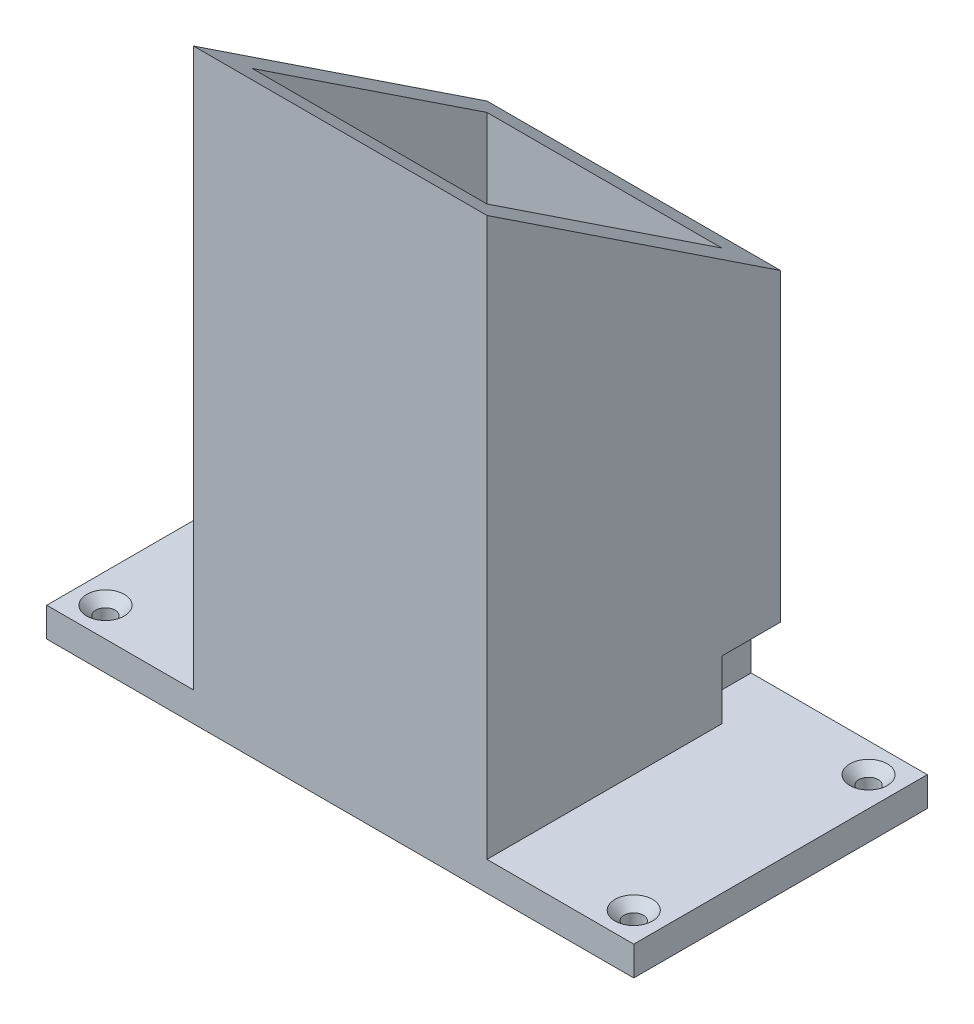
SolidWorks part; units mm, degrees
ref_plane "Front Plane" through (0, 0, 0) normal (0, 0, 1) x (1, 0, 0)
ref_plane "Top Plane" through (0, 0, 0) normal (0, 1, 0) x (1, 0, 0)
ref_plane "Right Plane" through (0, 0, 0) normal (1, 0, 0) x (0, 0, -1)
sketch "Sketch1" plane through (0, 0, 0) normal (0, 0, 1) x (1, 0, 0)
  line L0 (-100, -100) -> (-100, -90)
  line L5 (-50, 100) -> (50, 100)
  line L6 (-50, 100) -> (-50, -100)
  line L7 (-50, -100) -> (50, -100)
  line L8 (50, 100) -> (50, -100)
  line L9 (0, -100) -> (0, 100) construction
  line L10 (-50, 0) -> (50, 0) construction
  line L11 (50, -100) -> (100, -100)
  line L13 (50, -90) -> (100, -90)
  line L14 (100, -100) -> (100, -90)
  line L15 (-50, -100) -> (-100, -100)
  line L16 (-50, -90) -> (-100, -90)
  point P0 (0, 0)
  dimension "D1" = 200
  dimension "D2" = 100
  dimension "D3" = 50
  dimension "D4" = 10
extrude "Boss-Extrude1" add sketch "Sketch1" along normal blind 100 contours L6 L16 L0 L15 | L8 L5 L6 L7 | L11 L14 L13 L8
sketch "Sketch5" plane through (0, 0, 0) normal (1, 0, 0) x (0, 0, -1)
  line L0 (-100, 100) -> (0, 33.7713)
  line L1 (0, 100) -> (0, -90) construction
extrude "Cut-Extrude1" cut sketch "Sketch5" against normal through all and the other way through all
sketch "Sketch7" plane through (0, 0, 0) normal (0, 1, 0) x (1, 0, 0)
  line L0 (-50, -50) -> (50, -50) construction
  line L1 (-50, 0) -> (-50, -100) construction
  line L2 (50, -100) -> (50, 0) construction
  line L3 (0, 0) -> (0, -100) construction
  line L4 (-50, -100) -> (50, -100) construction
  line L5 (50, 0) -> (50, -100) construction
  line L6 (-40, -10) -> (40, -10)
  line L7 (-40, -10) -> (-40, -90)
  line L8 (-40, -90) -> (40, -90)
  line L9 (40, -10) -> (40, -90)
  line L10 (0, -90) -> (0, -10) construction
  line L11 (-40, -50) -> (40, -50) construction
  point P11 (0, -50)
  dimension "D1" = 10
  dimension "D2" = 10
extrude "Cut-Extrude2" cut sketch "Sketch7" against normal mid plane 200
sketch "Sketch8" plane through (0, 0, 0) normal (0, 0, -1) x (-1, 0, 0)
  line L0 (50, 33.7713) -> (50, -90) construction
  line L2 (50, -90) -> (100, -90) construction
  circle A0 centre (0, -40) radius 20
  dimension "D2" = 40
  dimension "D1" = 50
  dimension "D3" = 50
extrude "Cut-Extrude3" cut sketch "Sketch8" against normal blind 20
sketch "Sketch9" plane through (50, 0, 0) normal (1, 0, 0) x (0, 0, -1)
  line L0 (-50, 66.8857) -> (-50, -100) construction
  line L5 (0, 33.7713) -> (-100, 100) construction
  line L6 (-100, -100) -> (0, -100) construction
ref_plane "Plane1" [suppressed] through (0, 0, 50) normal (0, 0, -1) x (-1, 0, 0)
hole_wizard "CSK for M6 Hexagon lobular socket raised CTSK head screws1" positions "Sketch11" profile "Sketch12" countersink size "M6" standard "GB" end condition through all
sketch "Sketch11" plane through (0, -90, 0) normal (0, 1, 0) x (1, 0, 0)
  line L0 (-50, 0) -> (-100, 0) construction
  line L1 (-100, -100) -> (-100, 0) construction
  line L2 (-50, -100) -> (-100, -100) construction
  line L3 (100, -100) -> (100, 0) construction
  line L4 (50, 0) -> (100, 0) construction
  line L5 (50, -100) -> (100, -100) construction
  point P0 (-90, -10)
  point P2 (-90, -90)
  point P4 (90, -10)
  point P6 (90, -90)
  dimension "D1" = 10
  dimension "D2" = 10
  dimension "D3" = 10
  dimension "D4" = 10
  dimension "D5" = 10
  dimension "D6" = 10
  dimension "D7" = 10
  dimension "D8" = 10
sketch "Sketch12" plane through (-90, -90, 10) normal (1, 0, 0) x (0, 0, 1)
  line L0 (0, 0) -> (0, 10)
  line L1 (0, 10) -> (3.3, 10)
  line L2 (3.3, 10) -> (3.3, 3.1)
  line L3 (3.3, 3.1) -> (6.4, 0)
  line L5 (6.4, 0) -> (0, 0)
  line L6 (-3.3, 3.1) -> (-6.4, 0) construction
  line L11 (0, -6.35) -> (0, 107.95) construction
  dimension "通孔孔直径" = 6.6
  dimension "通孔孔深度" = 10
  dimension "近端锥形沉头孔直径" = 12.8
  dimension "近端锥形沉头孔角度" = 90
ref_plane "Plane2" [suppressed] through (0, 0, 0) normal (1, 0, 0) x (0, 0, -1)
ref_plane "Plane3" [suppressed] through (0, 0, 50) normal (0, 0, -1) x (-1, 0, 0)
sketch "Sketch13" plane through (50, 0, 0) normal (1, 0, 0) x (0, 0, -1)
  line L1 (0, -90) -> (-20, -90)
  line L2 (0, -90) -> (0, -70)
  line L3 (0, -70) -> (-20, -70)
  line L4 (-20, -90) -> (-20, -70)
  dimension "D1" = 20
  dimension "D2" = 20
extrude "Cut-Extrude4" cut sketch "Sketch13" against normal blind 10
